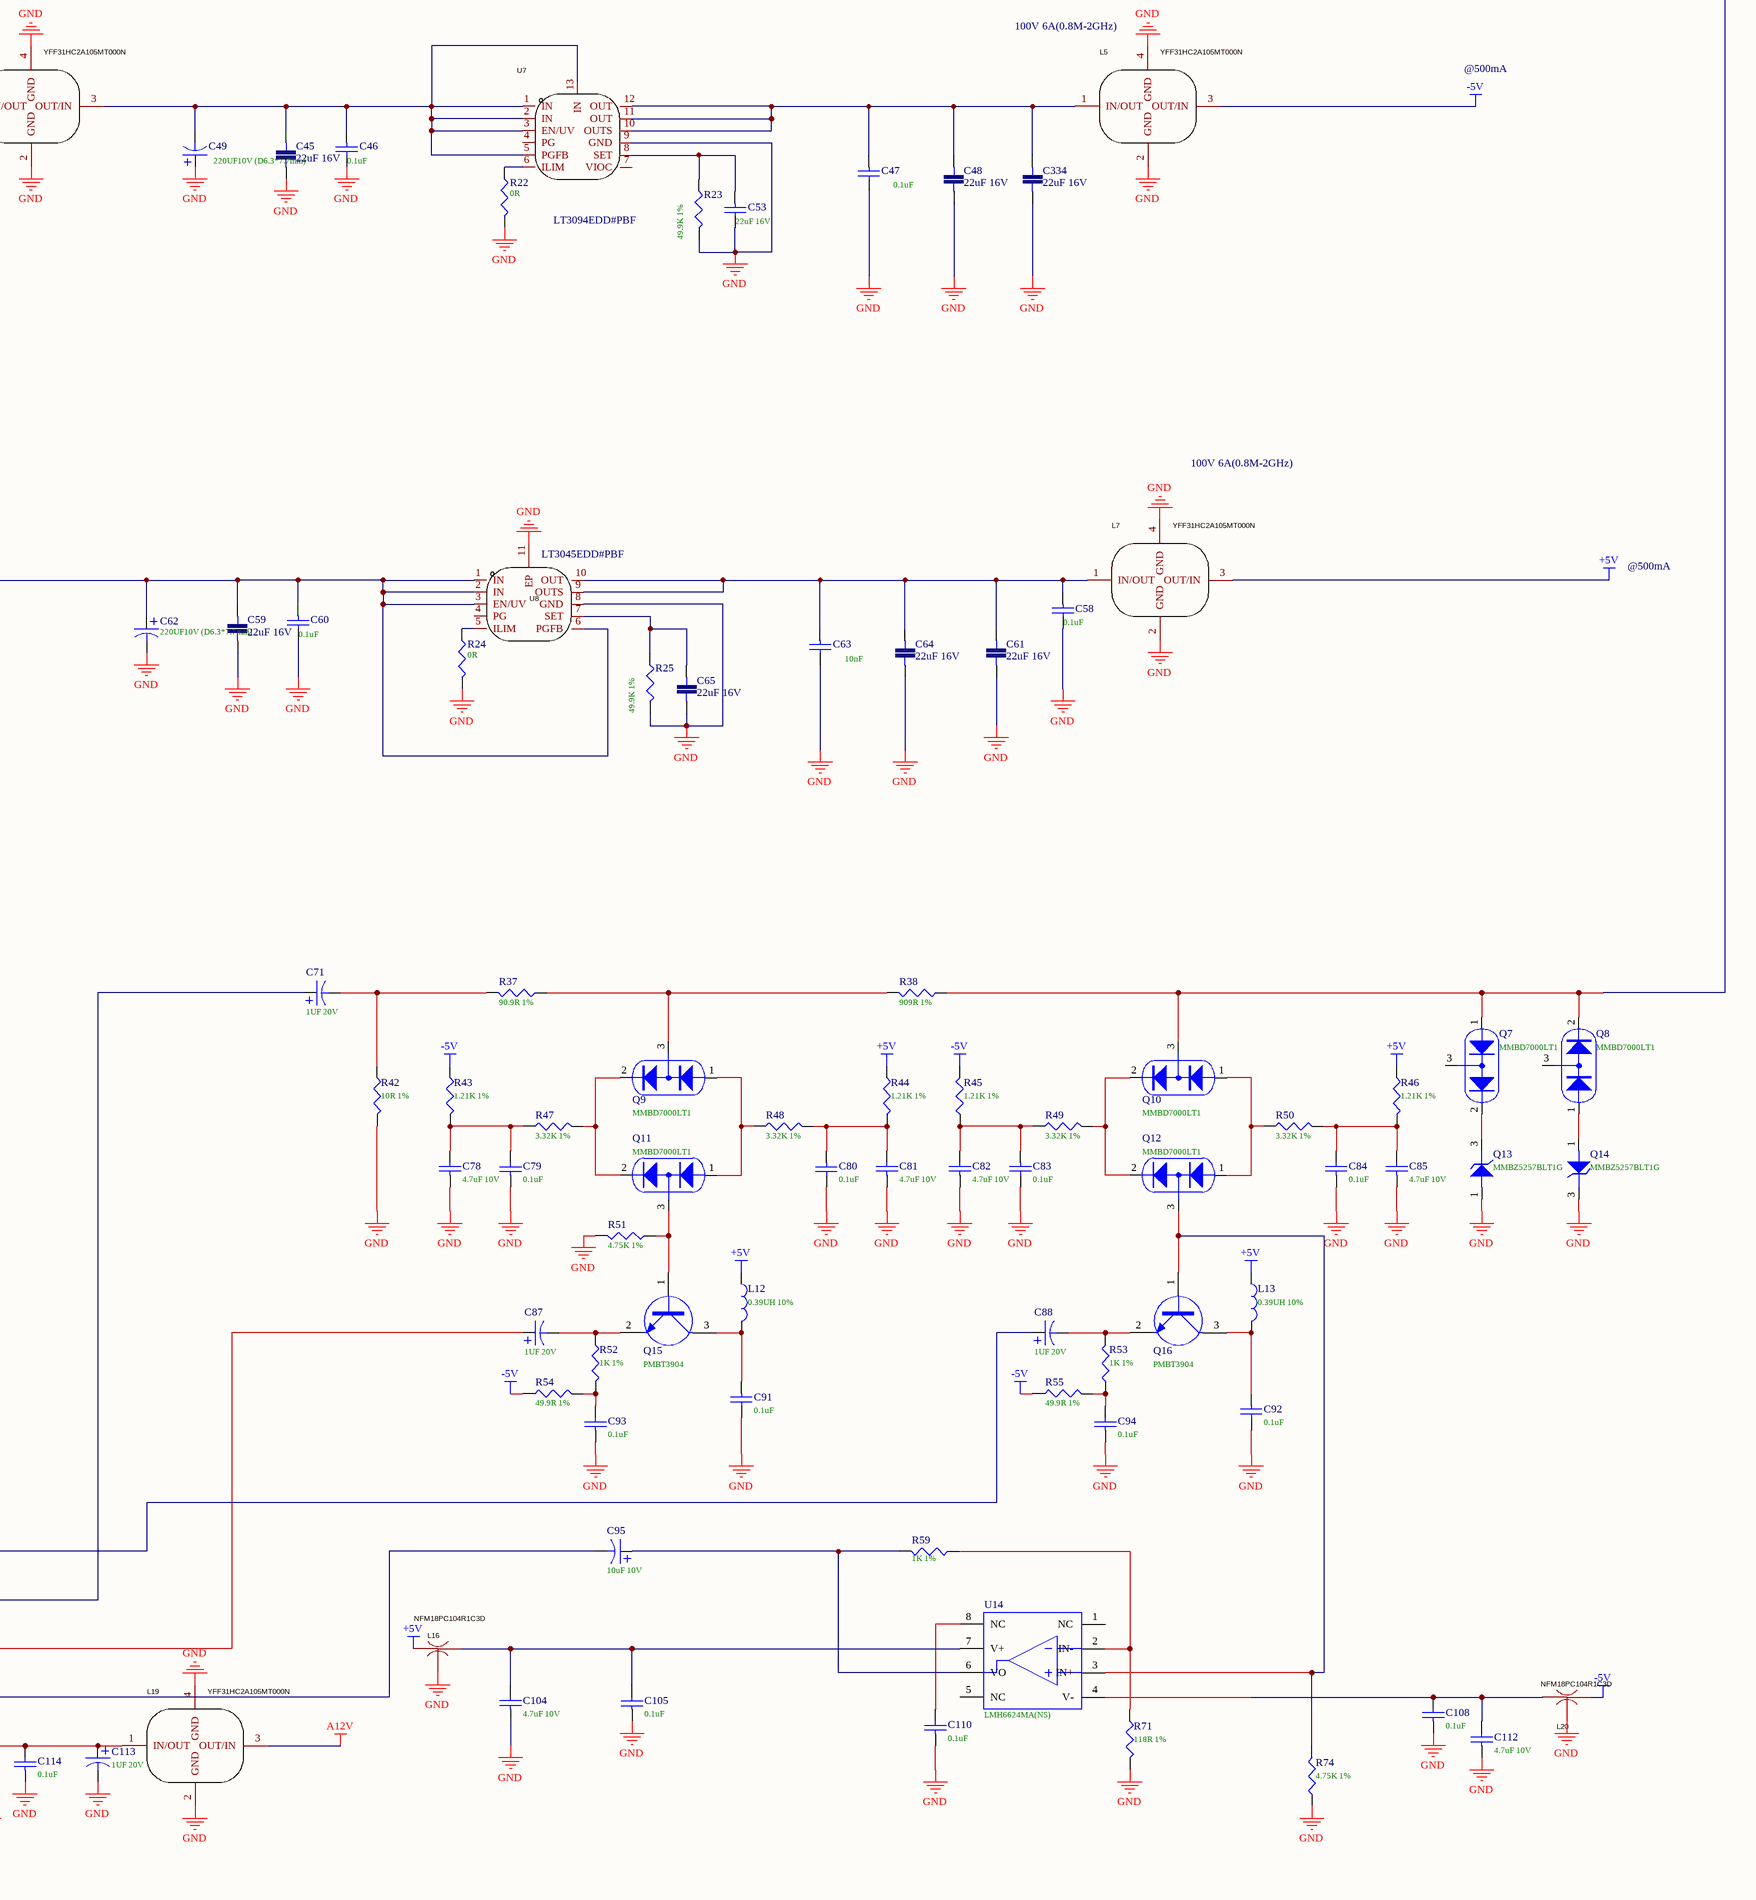
[diagram p0: PCBE109358.SchDoc, bottom column 3 of 4]
# Altium project MISC109358-2.PrjPcb (part 2 of 2)

## Sheet PCBE109358.SchDoc
size 1651 x 889 mm; SheetNumber: 0; SheetTotal: 0

### Parts
1  (no value)  [DIP-1]
+1  (no value)  [DIP-1]
+2  (no value)  [DIP-1]
C3  47uF 25V  [1206]
C4  0.1uF  [0402]
C5  1uF 25V  [0402]
C6  1uF 25V  [0402]
C7  47uF 25V  [1206]
C8  0.1uF  [0402]
C9  1uF 25V  [0402]
C14  0.1uF  [0402]
C15  47uF 25V  [1206]
C16  10uF 10V  [0603]
C17  10uF 10V  [0603]
C18  0.1uF 5% 630V  [AXIAL0.59]
C20  10uF 10V  [0603]
C21  10uF 10V  [0603]
C22  10nF  [0603]
C23  22uF 16V  [0603]
C24  0.1uF  [0603]
C25  0.1uF  [0402]
C26  22uF 16V  [0603]
C27  0.1uF  [0603]
C28  0.1uF  [0402]
C29  47uF 25V  [1206]
C30  47uF 25V  [1206]
C31  4.7uF 25V  [0603]
C32  0.1uF  [0402]
C33  47uF 25V  [1206]
C34  0.1uF  [0402]
C35  4.7uF 25V  [0603]
C36  0.1uF  [0402]
C37  0.1uF  [0402]
C38  4.7uF 10V  [0402]
C39  47uF 25V  [1206]
C40  0.1uF  [0402]
C41  0.1uF  [0402]
C42  47uF 25V  [1206]
C43  0.1uF  [0603]
C45  22uF 16V  [0603]
C46  0.1uF  [0402]
C47  0.1uF  [0402]
C48  22uF 16V  [0603]
C49  220UF10V (D6.3*7.7mm)  [CAP-SMD_BD6.3-L6.6-W6.6-FD]
C50  0.1uF  [0603]
C51  47uF 25V  [1206]
C53  22uF 16V  [0603]
C54  0.1uF  [0603]
C55  47uF 25V  [1206]
C56  2.2UF 10V  [0603钽电容]
C57  10pF  [0402]
C58  0.1uF  [0402]
C59  22uF 16V  [0603]
C60  0.1uF  [0402]
C61  22uF 16V  [0603]
C62  220UF10V (D6.3*7.7mm)  [CAP-SMD_BD6.3-L6.6-W6.6-FD]
C63  10nF  [0402]
C64  22uF 16V  [0603]
C65  22uF 16V  [0603]
C66  4.7uF 10V  [0402]
C67  0.1uF  [0402]
C68  4.7uF 10V  [0402]
C69  0.1uF  [0402]
C70  10nF  [0603]
C71  1UF 20V  [0603钽电容]
C72  NC  [0603]
C73  0.1uF  [0402]
C74  0.1uF  [0402]
C75  4.7uF 10V  [0402]
C76  0.1uF  [0402]
C77  4.7uF 10V  [0402]
C78  4.7uF 10V  [0402]
C79  0.1uF  [0402]
C80  0.1uF  [0402]
C81  4.7uF 10V  [0402]
C82  4.7uF 10V  [0402]
C83  0.1uF  [0402]
C84  0.1uF  [0402]
C85  4.7uF 10V  [0402]
C86  10pF  [0402]
C87  1UF 20V  [0603钽电容]
C88  1UF 20V  [0603钽电容]
C89  4.7uF 10V  [0402]
C90  0.1uF  [0402]
C91  0.1uF  [0402]
C92  0.1uF  [0402]
C93  0.1uF  [0402]
C94  0.1uF  [0402]
C95  10uF 10V  [0603钽电容]
C96  NC  [0603]
C97  0.1uF  [0402]
C98  2.2nF 1%  [0402]
C99  0.1uF  [0402]
C100  4.7uF 10V  [0402]
C101  0.1uF  [0402]
C102  4.7uF 10V  [0402]
C103  2.2nF 1%  [0402]
C104  4.7uF 10V  [0402]
C105  0.1uF  [0402]
C106  1.2nF 1%  [0402]
C107  0.1uF  [0402]
C108  0.1uF  [0402]
C109  2.2UF 10V  [0603钽电容]
C110  0.1uF  [0603]
C111  270pF 1%  [0603]
C112  4.7uF 10V  [0402]
C113  1UF 20V  [0603钽电容]
C114  0.1uF  [0402]
C115  0.1uF  [0402]
C116  0.1uF  [0402]
C117  4.7uF 10V  [0402]
C118  0.1uF  [0402]
C119  100pF 1%  [0603]
C120  4.7uF 10V  [0402]
C121  0.1uF  [0402]
C122  4.7uF 10V  [0402]
C123  4.7uF 10V  [0402]
C124  0.1uF  [0402]
C125  56pF 1%  [0603]
C126  0.1uF  [0402]
C127  4.7uF 10V  [0402]
C128  0.1uF  [0402]
C129  4.7uF 10V  [0402]
C301  0.1uF  [0402]
C302  0.1uF  [0402]
C304  0.1uF  [0402]
C305  4.7uF 10V  [0402]
C306  0.1uF  [0402]
C307  4.7uF 10V  [0402]
C334  22uF 16V  [0603]
D1  ES1D SMA  [1606D]
D2  MMBD914LT1G  [SOT23]
D3  MMBD914LT1G  [SOT23]
D4  ES1D SMA  [1606D]
D5  3SMAJ5929B  [1606D]
D6  DFLU1400-7  [1606D]
D7  ES1D SMA  [1606D]
D8  MMBD914LT1G  [SOT23]
D9  MMBD914LT1G  [SOT23]
D10  MMSZ5248B  [1206D]
D11  MMBZ5231B  [SOT23]
J1  RF connector right-angle socket  [DIP-P]
J2  RF connector right-angle socket  [DIP-P]
K1  TQ2SS-5V(ATQ209SS)SMD10  [K]
K2  TQ2SS-5V(ATQ209SS)SMD10  [K]
K3  TQ2SS-5V(ATQ209SS)SMD10  [K]
K4  TQ2SS-5V(ATQ209SS)SMD10  [K]
L1  YFF31HC2A105MT000N  [FILTER-SMD_4P-L3.2-W1.6-L_YFF31HC]
L2  YFF31HC2A105MT000N  [FILTER-SMD_4P-L3.2-W1.6-L_YFF31HC]
L3  YFF31HC2A105MT000N  [FILTER-SMD_4P-L3.2-W1.6-L_YFF31HC]
L4  YFF31HC2A105MT000N  [FILTER-SMD_4P-L3.2-W1.6-L_YFF31HC]
L5  YFF31HC2A105MT000N  [FILTER-SMD_4P-L3.2-W1.6-L_YFF31HC]
L6  YFF31HC2A105MT000N  [FILTER-SMD_4P-L3.2-W1.6-L_YFF31HC]
L7  YFF31HC2A105MT000N  [FILTER-SMD_4P-L3.2-W1.6-L_YFF31HC]
L8  NFM18PC104R1C3D  [FILTER-SMD_3P-L1.6-W0.8-L_NFM18CC223R1C3D]
L9  NFM18PC104R1C3D  [FILTER-SMD_3P-L1.6-W0.8-L_NFM18CC223R1C3D]
L10  NFM18PC104R1C3D  [FILTER-SMD_3P-L1.6-W0.8-L_NFM18CC223R1C3D]
L11  NFM18PC104R1C3D  [FILTER-SMD_3P-L1.6-W0.8-L_NFM18CC223R1C3D]
L12  0.39UH 10%  [0805]
L13  0.39UH 10%  [0805]
L14  NFM18PC104R1C3D  [FILTER-SMD_3P-L1.6-W0.8-L_NFM18CC223R1C3D]
L15  NFM18PC104R1C3D  [FILTER-SMD_3P-L1.6-W0.8-L_NFM18CC223R1C3D]
L16  NFM18PC104R1C3D  [FILTER-SMD_3P-L1.6-W0.8-L_NFM18CC223R1C3D]
L17  NFM18PC104R1C3D  [FILTER-SMD_3P-L1.6-W0.8-L_NFM18CC223R1C3D]
L18  NFM18PC104R1C3D  [FILTER-SMD_3P-L1.6-W0.8-L_NFM18CC223R1C3D]
L19  YFF31HC2A105MT000N  [FILTER-SMD_4P-L3.2-W1.6-L_YFF31HC]
L20  NFM18PC104R1C3D  [FILTER-SMD_3P-L1.6-W0.8-L_NFM18CC223R1C3D]
L21  NFM18PC104R1C3D  [FILTER-SMD_3P-L1.6-W0.8-L_NFM18CC223R1C3D]
L22  18UH 5%  [0805]
L23  NFM18PC104R1C3D  [FILTER-SMD_3P-L1.6-W0.8-L_NFM18CC223R1C3D]
L24  NFM18PC104R1C3D  [FILTER-SMD_3P-L1.6-W0.8-L_NFM18CC223R1C3D]
L25  10UH 5%  [0805]
L26  NFM18PC104R1C3D  [FILTER-SMD_3P-L1.6-W0.8-L_NFM18CC223R1C3D]
L27  3.9UH 5%  [0805]
L60  NFM18PC104R1C3D  [FILTER-SMD_3P-L1.6-W0.8-L_NFM18CC223R1C3D]
L61  NFM18PC104R1C3D  [FILTER-SMD_3P-L1.6-W0.8-L_NFM18CC223R1C3D]
P1  Header 20X2  [N0.8mm/40Pin-Plug]
P2  Header 4X2  [N0.8mm/8Pin-SOCKET]
P4  Header 20X2  [N0.8mm/40Pin-Plug]
P5  Header 20X2  [N0.8mm/40Pin-Plug]
P6  RF connector straight jack  [DIP-P]
P9  RF connector straight jack  [DIP-P]
Q1  PMBT3904  [SOT23]
Q2  STP10NK80Z  [TO220]
Q3  PMBT3904  [SOT23]
Q4  2N7002-7-F  [SOT23]
Q5  MMBD914LT1G  [SOT23]
Q6  MMBD914LT1G  [SOT23]
Q7  MMBD7000LT1  [SOT23]
Q8  MMBD7000LT1  [SOT23]
Q9  MMBD7000LT1  [SOT23]
Q10  MMBD7000LT1  [SOT23]
Q11  MMBD7000LT1  [SOT23]
Q12  MMBD7000LT1  [SOT23]
Q13  MMBZ5257BLT1G  [SOT23]
Q14  MMBZ5257BLT1G  [SOT23]
Q15  PMBT3904  [SOT23]
Q16  PMBT3904  [SOT23]
Q17  BFT92  [SOT23]
R1  0R  [0402]
R2  470R 5% 1W  [2512]
R3  1K 1W  [2512]
R4  1K 1W  [2512]
R5  2.21K 1%  [0603]
R6  220R 5% 1W  [2512]
R7  10K 1%  [0603]
R8  1.5R  [0603]
R9  1.15K 1%  [1206]
R10  0.5R 1%  [0805]
R11  52.5K 1%  [0603]
R12  1.5R  [0603]
R13  2.21K 1%  [0603]
R14  82R 5% 3W  [2512]
R15  10K 1%  [0603]
R16  10K 1%  [0603]
R17  10K 1%  [0603]
R18  51R 5W  [5W]
R19  13.3K  1%  [0402]
R20  121K  [0603]
R21  0R  [0402]
R22  0R  [0402]
R23  49.9K 1%  [0402]
R24  0R  [0402]
R25  49.9K 1%  [0402]
R26  47R 1%  [0603]
R27  681R 1%  [0603]
R28  22.1K 1%  [0603]
R29  10R 1%  [0603]
R30  100R 1%  [0603]
R31  100R 1%  [0603]
R32  681R 1%  [0603]
R33  0R  [0402]
R34  1K 1%  [0603]
R35  681R 1%  [0603]
R36  100R 1%  [0603]
R37  90.9R 1%  [1206]
R38  909R 1%  [1206]
R39  1.21K 1%  [0603]
R40  5.62K 1%  [0603]
R41  10K 1%  [0603]
R42  10R 1%  [0603]
R43  1.21K 1%  [0603]
R44  1.21K 1%  [0603]
R45  1.21K 1%  [0603]
R46  1.21K 1%  [0603]
R47  3.32K 1%  [0603]
R48  3.32K 1%  [0603]
R49  3.32K 1%  [0603]
R50  3.32K 1%  [0603]
R51  4.75K 1%  [0603]
R52  1K 1%  [0603]
R53  1K 1%  [0603]
R54  49.9R 1%  [0603]
R55  49.9R 1%  [0603]
R56  100R 1%  [0603]
R57  301R 1%  [0603]
R58  20R 1%  [0603]
R59  1K 1%  [0603]
R60  20K 1%  [0603]
R61  20K 1%  [0603]
R62  1K 1%  [0603]
R63  1.21K 1%  [0603]
R64  100R 1%  [0603]
R65  20K 1%  [0603]
R66  1K 1%  [0603]
R67  22.1K 1%  [0603]
R68  0R  [0402]
R69  20K 1%  [0603]
R70  10R 1%  [0603]
R71  118R 1%  [0603]
R72  0R  [0603]
R73  20R 1%  [0603]
R74  4.75K 1%  [0603]
R75  5.62K 1%  [0603]
R76  1K 1%  [0603]
R77  49.9R 1%  [0603]
R78  1.21K 1%  [0603]
R79  10R 1%  [0603]
R800  523K 1%  [0402]
R801  4.7K 1%  [0402]
TP1  (no value)  [TP1]
U1  TPS7A4701RGWR  [QFN-20]
U2  TC4426COA(microchip)  [SO8]
U3  TPL910A  [DFN-8_L3.0-W3.0-P0.65-BL-EP2.3]
U4  TC4426COA(microchip)  [SO8]
U5  GM12051ACPZ-R7  [TDFN-10_L3.0-W3.0-P0.50-BL-EP]
U6  ADR391AUJZ-REEL7  [TSOT-23-5_L2.9-W1.6-P0.95-LS2.8-BR]
U7  LT3094EDD#PBF  [WDFN-12_L3.0-W3.0-P0.45-BL-EP]
U8  LT3045EDD#PBF  [DFN-10_L3.0-W3.0-P0.50-BL-EP]
U9  MASWSS0157TR  [SO8]
U10  AD603AR  [SO8]
U11  AD8002ARZ  [SOP8]
U12  SN74AHC1G04DBVR  [SOT25]
U13  DG540DN PLCC20  [QUAD20]
U14  LMH6624MA(NS)  [SO8]
U15  ADG658YRQZ  [TSSOP-16_L5.0-W4.4-P0.65-LS6.4-TL]
U16  ADG658YRQZ  [TSSOP-16_L5.0-W4.4-P0.65-LS6.4-TL]
U17  AD603AR  [SO8]
U60  AD8002ARZ  [SOP8]

### Nets
12.4V: +2.1 C3.1 C4.1 C5.1 C34.1 C35.1 C54.1 C55.1 L2.3(OUT/IN) P5.31 P5.32 P5.33 P5.34 P5.35 P5.36 P5.37 P5.38 P5.39 P5.40 U1.13(EN) U1.15(IN) U1.16(IN)
+5V: L3.1(IN/OUT) L7.3(OUT/IN) L8.3(OUTPUT) L9.1(INPUT) L12.1 L13.1 L15.1(INPUT) L16.1(INPUT) L17.1(INPUT) L24.3(OUTPUT) L60.3(OUTPUT) R44.1 R46.1 R58.1
-5.4V: +1.1 C42.1 C43.1 L4.1(IN/OUT) P5.1 P5.2 P5.3 P5.4 P5.5 P5.6 P5.7 P5.8 P5.9 P5.10
-5V: L5.3(OUT/IN) L10.1(INPUT) L11.3(OUTPUT) L14.1(INPUT) L18.3(OUTPUT) L20.3(OUTPUT) L21.1(INPUT) L23.1(INPUT) L26.1(INPUT) L61.3(OUTPUT) R43.2 R45.1 R54.2 R55.1 R73.2
A6V: 1.1 C23.2 C24.1 C50.2 C51.1 L6.1(IN/OUT) P5.17 P5.18 P5.19 P5.20 P5.21 P5.22 P5.23 P5.24 U3.5(EN) U3.7(IN) U3.8(IN)
A12V: C30.1 C36.1 C37.1 L19.3(OUT/IN) R801.1 U5.9(OUTS) U5.10(OUT)
GND: C3.2 C4.2 C5.2 C6.2 C7.2 C8.2 C9.2 C14.2 C15.2 C16.1 C17.1 C20.1 C21.1 C23.1 C24.2 C25.2 C26.2 C27.2 C28.2 C29.2 C30.2 C31.2 C32.2 C33.2 C34.2 C35.2 C36.2 C37.2 C38.1 C39.2 C40.1 C41.1 C42.2 C43.2 C45.1 C46.2 C47.2 C48.1 C49.1 C50.1 C51.2 C53.2 C54.2 C55.2 C57.1 C58.2 C59.1 C60.2 C61.1 C62.2 C63.2 C64.1 C65.1 C66.1 C67.2 C68.1 C69.2 C72.2 C73.2 C74.2 C75.1 C76.2 C77.1 C78.1 C79.1 C80.2 C81.1 C82.1 C83.2 C84.1 C85.1 C86.2 C89.1 C90.2 C91.2 C92.2 C93.1 C94.1 C96.2 C97.1 C99.1 C100.1 C101.2 C102.1 C103.1 C104.1 C105.1 C108.1 C110.1 C112.1 C113.2 C114.1 C115.2 C116.1 C117.1 C118.1 C120.1 C121.1 C122.1 C123.1 C124.2 C126.1 C127.1 C128.1 C129.1 C301.2 C302.1 C304.2 C305.1 C306.2 C307.1 C334.1 D10.1(A) J1.1 J1.2 J1.3 J1.4 J2.1 J2.2 J2.3 J2.4 K1.3 K1.8 K2.4 K2.7 K3.3 K3.8 K4.4 K4.7 L1.2(GND) L1.4(GND) L2.2(GND) L2.4(GND) L3.2(GND) L3.4(GND) L4.2(GND) L4.4(GND) L5.2(GND) L5.4(GND) L6.2(GND) L6.4(GND) L7.2(GND) L7.4(GND) L8.2(GND) L9.2(GND) L10.2(GND) L11.2(GND) L14.2(GND) L15.2(GND) L16.2(GND) L17.2(GND) L18.2(GND) L19.2(GND) L19.4(GND) L20.2(GND) L21.2(GND) L23.2(GND) L24.2(GND) L26.2(GND) L60.2(GND) L61.2(GND) P1.5 P1.6 P1.11 P1.12 P1.17 P1.18 P1.20 P1.23 P1.24 P1.29 P1.30 P1.35 P1.36 P2.1 P2.3 P2.5 P2.7 P4.5 P4.6 P4.11 P4.12 P4.17 P4.18 P4.23 P4.24 P4.29 P4.30 P4.35 P4.36 P5.11 P5.12 P5.13 P5.14 P5.15 P5.16 P5.25 P5.26 P5.27 P5.28 P5.29 P5.30 P6.1 P6.2 P6.3 P6.4 P9.1 P9.2 P9.3 P9.4 Q1.2(E) Q3.2(E) Q4.2(S) Q5.3(K) Q6.1(A) Q13.1(A) Q14.3(K) R2.2 R7.2 R9.2 R10.1 R15.2 R16.2 R17.1 R19.2 R20.2 R21.2 R22.2 R23.2 R24.2 R25.2 R34.2 R35.2 R36.2 R39.2 R40.1 R41.1 R42.1 R51.2 R60.1 R61.2 R63.1 R65.2 R66.1 R69.1 R71.1 R74.1 R75.1 R78.2 U1.5(6P4V1) U1.6(3P2V) U1.7(GND) U1.9(0P8V) U1.11(0P2V) U1.21(EPAD) U2.3(GND) U3.4(GND) U3.9(pad) U4.3(GND) U5.8(GND) U5.11(EP) U6.5(GND) U7.9(GND) U8.8(GND) U8.11(EP) U9.2(GND) U9.7(GND) U9.8(GND) U10.4(COMM) U12.5(VCC) U13.3(GND) U13.6(GND) U13.8(GND) U13.13(GND) U13.15(GND) U13.18(GND) U15.6(EN#) U15.8(GND) U16.6(EN#) U16.8(GND) U17.4(COMM)
H5V: C16.2 C17.2 C20.2 C21.2 C22.2 C25.1 C26.1 D2.3(K) D3.3(K) D8.3(K) D9.3(K) K1.1 K2.1 K3.1 K4.1 R11.2 TP1.1 U3.1(OUT) U3.2(OUT)
H12V: C7.1 C8.1 C9.1 D1.2(K) L1.1(IN/OUT) R1.1 U1.1(OUT) U1.20(OUT)
VREF: C38.2 C41.2 R28.1 R67.2 U6.3(VOUT/SENSE) U6.4(VOUT/FORCE)
AK1: P1.27 Q4.1(G) R17.2
AK10: P1.19 R13.2
AK13: P1.21 R5.2
AS27: P4.38
AS28: P4.40
Attn1: P4.34
Attn2: P4.32
Attn4: P4.28
Attn8: P4.26
Attn16: P4.22
DAC Clk: P4.14
DAC Data: P4.16
DAC Strobe: P4.10
GPOS1: C72.1 C96.1 R56.1 U10.1(GPOS) U17.1(GPOS)
HP Filt En: P4.4
HT: P2.2 P2.4 P2.6 P2.8 R3.2
IN1: P4.20
IN2: P4.8
K0: D11.3(K) P4.9
LB_A0: P4.27 U15.9(A2)
LB_A1: P4.25 U15.10(A1)
LB_A2: P4.21 U15.11(A0)
LB_A4: P4.19 U16.9(A2)
LB_A5: P4.15 U16.10(A1)
LB_A6: P4.13 U16.11(A0)
LB_IN1: R72.1 U15.13(S1)
LB_IN2: R77.2 U15.14(S2)
LB_IN3: R79.2 U15.15(S3)
LB_IN4: R68.1 U15.12(S4)
LB_OUT: R33.1 R41.2 U16.3(D)
LP Filt En: P4.2
TT: P1.22 R9.1 U2.2(IN_A) U2.4(IN_B) U4.2(IN_A) U4.4(IN_B)
U15_IN1: P4.39 R61.1 U13.20(IN2)
U15_IN2: P4.37 R60.2 U13.1(IN1)
U15_IN3: P4.33 R65.1 U13.11(IN3)
U15_IN4: P4.31 R69.2 U13.10(IN4)
NetC6_1: C6.1 U1.14(NR)
NetC14_1: C14.1 C15.1 C28.1 C29.1 L1.3(OUT/IN) U2.6(VDD) U4.6(VDD)
NetC18_1: C18.1 Q2.2(D) R4.2
NetC18_2: C18.2 D5.2(K) D6.2(K)
NetC22_1: C22.1 R11.1 R15.1 U3.3(FB)
NetC27_1: C27.1 U3.6(RN)
NetC31_1: C31.1 R20.1 U5.7(SET)
NetC32_1: C32.1 C33.1 L2.1(IN/OUT) U5.1(IN) U5.2(IN) U5.3(EN/UV)
NetC39_1: C39.1 C40.2 L3.3(OUT/IN) U6.1(SHDN#) U6.2(VIN)
NetC45_2: C45.2 C46.1 C49.2 L4.3(OUT/IN) U7.1(IN) U7.2(IN) U7.3(EN/UV) U7.5(PGFB) U7.13(IN)
NetC47_1: C47.1 C48.2 C334.2 L5.1(IN/OUT) U7.10(OUTS) U7.11(OUT) U7.12(OUT)
NetC53_1: C53.1 R23.1 U7.8(SET)
NetC56_1: C56.1 C57.2 P6.5
NetC56_2: C56.2 Q5.1(A) Q6.3(K) R26.2
NetC58_1: C58.1 C61.2 C63.1 C64.2 L7.1(IN/OUT) U8.9(OUTS) U8.10(OUT)
NetC59_2: C59.2 C60.1 C62.1 L6.3(OUT/IN) U8.1(IN) U8.2(IN) U8.3(EN/UV) U8.6(PGFB)
NetC65_2: C65.2 R25.1 U8.7(SET)
NetC66_2: C66.2 C67.1 L8.1(INPUT) U11.8(V+)
NetC68_2: C68.2 C69.1 L9.3(OUTPUT) U10.8(VPOS)
NetC70_1: C70.1 R39.1 U9.3(RF1)
NetC70_2: C70.2 R29.1
NetC71_1: C71.1 U13.17(S2)
NetC71_2: C71.2 R37.1 R42.2
NetC73_1: C73.1 R28.2 R40.2 U10.2(GNEG)
NetC74_1: C74.1 C75.2 L10.3(OUTPUT) U10.6(VNEG)
NetC76_1: C76.1 C77.2 L11.1(INPUT) U11.4(V-)
NetC78_2: C78.2 C79.2 R43.1 R47.2
NetC80_1: C80.1 C81.2 R44.2 R48.1
NetC82_2: C82.2 C83.1 R45.2 R49.1
NetC84_2: C84.2 C85.2 R46.2 R50.2
NetC86_1: C86.1 U9.4(A) U12.4(Y)
NetC87_1: C87.1 U13.14(S3)
NetC87_2: C87.2 Q15.2(E) R52.1
NetC88_1: C88.1 U13.4(S1)
NetC88_2: C88.2 Q16.2(E) R53.2
NetC89_2: C89.2 C90.1 L14.3(OUTPUT) U12.3(GND)
NetC91_1: C91.1 L12.2 Q15.3(C)
NetC92_1: C92.1 L13.2 Q16.3(C)
NetC93_2: C93.2 R52.2 R54.1
NetC94_2: C94.2 R53.1 R55.2
NetC95_1: C95.1 R59.2 U14.6(VO)
NetC95_2: C95.2 U13.7(S4)
NetC97_2: C97.2 R57.2 R58.2
NetC98_1: C98.1 C106.1 U16.15(S3)
NetC98_2: C98.2 C103.2 C106.2 R68.2
NetC99_2: C99.2 C102.2 L17.3(OUTPUT) U17.8(VPOS)
NetC100_2: C100.2 C101.1 L15.3(OUTPUT) R62.2
NetC104_2: C104.2 C105.2 L16.3(OUTPUT) U14.7(V+)
NetC107_1: C107.1 U15.3(D)
NetC107_2: C107.2 R70.2
NetC108_2: C108.2 C112.2 L20.1(INPUT) U14.4(V-)
NetC109_1: C109.1 Q17.2(E) R57.1
NetC109_2: C109.2 U17.3(VINP)
NetC110_2: C110.2 U14.8(NC)
NetC111_1: C111.1 L22.1
NetC111_2: C111.2 R72.2
NetC113_1: C113.1 C114.2 L19.1(IN/OUT) U13.16(V+)
NetC115_1: C115.1 R67.1 R75.2 U17.2(GNEG)
NetC116_2: C116.2 C117.2 Q17.3(C) R73.1
NetC118_2: C118.2 C120.2 L21.3(OUTPUT) U13.5(V-)
NetC119_1: C119.1 L25.1
NetC119_2: C119.2 R77.1
NetC121_2: C121.2 C122.2 L26.3(OUTPUT) U17.6(VNEG)
NetC123_2: C123.2 C124.1 L23.3(OUTPUT) U16.7(VSS)
NetC125_1: C125.1 L27.1
NetC125_2: C125.2 R79.1
NetC126_2: C126.2 C129.2 L24.1(INPUT) R76.2
NetC127_2: C127.2 C128.2 L18.1(INPUT) U15.7(VSS)
NetC301_1: C301.1 R62.1 R63.2 U16.16(VDD)
NetC302_2: C302.2 R76.1 R78.1 U15.16(VDD)
NetC304_1: C304.1 C305.2 L61.1(INPUT) U60.4(V-)
NetC306_1: C306.1 C307.2 L60.1(INPUT) U60.8(V+)
NetD1_1: D1.1(A) D4.2(K)
NetD2_1: D2.1(A) K1.10 Q1.3(C)
NetD3_1: D3.1(A) D9.1(A) K2.10 K4.10 Q4.3(D)
NetD4_1: D4.1(A) D5.1(A)
NetD6_1: D6.1(A) D7.2(K)
NetD7_1: D7.1(A) J1.5 K2.2 K2.9 R2.1 R6.2 R14.2
NetD8_1: D8.1(A) K3.10 Q3.3(C)
NetD10_2: D10.2(K) Q2.1(G) R8.1 R12.1
NetD11_1: D11.1(A) U12.2(A)
NetJ2_5: J2.5 K4.2 K4.9 R18.1
NetK1_4: K1.4 K1.7 R6.1
NetK2_3: K2.3 K2.8 K4.3 K4.8
NetK3_4: K3.4 K3.7 R14.1
NetL22_2: L22.2 U16.14(S2)
NetL25_2: L25.2 U16.13(S1)
NetL27_2: L27.2 U16.12(S4)
NetP9_5: P9.5 R56.2
NetQ1_1: Q1.1(B) R5.1 R7.1
NetQ2_3: Q2.3(S) R10.2
NetQ3_1: Q3.1(B) R13.1 R16.1
NetQ7_1: Q7.1 Q8.2 Q10.3 R18.2 R38.2
NetQ7_2: Q7.2 Q13.3(K)
NetQ8_1: Q8.1 Q14.1(A)
NetQ9_1: Q9.1 Q11.1 R48.2
NetQ9_2: Q9.2 Q11.2 R47.1
NetQ9_3: Q9.3 R37.2 R38.1
NetQ10_1: Q10.1 Q12.1 R50.1
NetQ10_2: Q10.2 Q12.2 R49.2
NetQ11_3: Q11.3 Q15.1(B) R51.1
NetQ12_3: Q12.3 Q16.1(B) R74.2 U14.3(IN+)
NetQ17_1: Q17.1(B) R64.1
NetR1_2: R1.2 U1.3(SENSE/FB)
NetR3_1: R3.1 R4.1
NetR8_2: R8.2 U2.7(~{OUTA}) U4.7(~{OUTA})
NetR12_2: R12.2 U2.5(~{OUTB}) U4.5(~{OUTB})
NetR19_1: R19.1 R800.2 U5.6(PGFB)
NetR21_1: R21.1 U5.5(ILIM)
NetR22_1: R22.1 U7.6(ILIM)
NetR24_1: R24.1 U8.5(ILIM)
NetR26_1: R26.1 R27.1 U60.1(OUT1)
NetR27_2: R27.2 R35.1 U60.2(-IN1)
NetR29_2: R29.2 R32.1 U11.7(OUT2)
NetR30_1: R30.1 U60.3(+IN1)
NetR30_2: R30.2 R34.1 U9.1(RFC)
NetR31_1: R31.1 U11.5(+IN2)
NetR31_2: R31.2 U10.5(FDBK) U10.7(VOUT)
NetR32_2: R32.2 R36.1 U11.6(-IN2)
NetR33_2: R33.2 U10.3(VINP)
NetR59_1: R59.1 R71.2 U14.2(IN-)
NetR64_2: R64.2 R66.2 U13.2(D1) U13.9(D4) U13.12(D3) U13.19(D2)
NetR70_1: R70.1 U17.5(FDBK) U17.7(VOUT)
NetR800_1: R800.1 R801.2

Not connected (* = marked no-connect by the designer): K1 2 5 6 9; K2 5 6; K3 2 5 6 9; K4 5 6; P1 1 2 3 4 7 8 9 10 13 14 15 16 25 26 28 31 32 33 34 37 38 39 40; P4 1 3 7; Q7 3; Q8 3; U1 2(NC) 4(6P4V2) 8(1P6V) 10(0P4V) 12(0P1V) 17(NC) 18(NC) 19(NC); U2 1(NC) 8(NC); U4 1(NC) 8(NC); U5 4(PG); U7 4(PG) 7(VIOC); U8 4(PG); U9 5(B) 6(RF2); U11 1(OUT1) 2(-IN1) 3(+IN1); U14 1(NC) 5(NC); U15 1(S5) 2(S7) 4(S8) 5(S6); U16 1(S5) 2(S7) 4(S8) 5(S6); U60 5(+IN2) 6(-IN2) 7(OUT2)

### Notes on the sheet
- @1A
- (near P2) 500V high-voltage interface
- transmit interface
- (near U2) negative pulse
- (near R7) separate shield ring
- receive interface
- Couts connected to output capacitor and load
- (near L5) 100V 6A(0.8M-2GHz)
- @500mA
- 100V 6A(0.8M-2GHz)
- (near R68) 0.25MHz--2.25MHz
- tentative 2-10MHZ
- 2.25MHz
- (near R77) tentative 10-30MHZ
- (near R77) 5MHz
- (near R79) 10MHz(7.5--14.5MHz)
- Title
- Size:
- Date:
- File:
- A0
- Number:
- Time:
- Revision:
- Sheet
- of

### Library data of the parts
1 +1 +2 = TP
C3-C9 C14-C18 C20 C21 C28-C43 C46 C47 C50 C51 C53-C55 C57 C58 C60 C63 C66-C70 C72-C86 C89-C94 C96-C108 C110-C112 C114-C129 C301 C302 C304-C307 = CAP: Capacitor
C22 C23 C25 C26 C45 C48 C59 C61 C64 C65 C334 = C1206
C24 C27 = C0402
C49 C62 = CAPACITOR_1: Capacitor
C56 C71 C87 C88 C95 C109 C113 = CAPACITOR
D1 D4 D6 D7 = DIODE
D5 D10 = ZENER3: Zener Diode
D11 = MMBZ5257BLT1G
J1 J2 P6 P9 = JA1
K1-K4 = TQ2SS-5V
L1-L7 L19 = YFF31HC2A105MT000N: Manufacturer: TDK; Add into BOM: yes; Nominal Capacitance: 1uF; CapacitanceTolerance: ±20%; DC Rated Voltage: 100V; Rated Current: 6A; DC Resistance: 5mΩ; Name: YFF31HC2A105MT000N; Symbol: YFF31HC2A105MT000N; Device: YFF31HC2A105MT000N; LCSC Part Name: 1uF(105) ±20% 100V; Supplier Part: C113216; Manufacturer Part: YFF31HC2A105MT000N; Supplier Footprint: SMD-4P,1.6x3.2mm; JLCPCB Part Class: Extended Part; Datasheet: https://example.com/upload/public/pdf/source/20180326/C113216_F6F81E50B9805DA3D7C436129903DEBD.pdf; Supplier: LCSC; Convert to PCB: yes; Operating Temperature: -55℃~+125℃
L8-L11 L14-L18 L20 L21 L23 L24 L26 L60 L61 = NFM15PC104R1A3D: Manufacturer: muRata(村田); Add into BOM: yes; Nominal Capacitance: 100nF; CapacitanceTolerance: ±20%; DC Rated Voltage: 10V; Rated Current: 2A; DC Resistance: 30mΩ; Symbol: NFM15PC104R1A3D; Device: NFM15PC104R1A3D; LCSC Part Name: 0.1uF ±20% 10V; Supplier Part: C2650905; Manufacturer Part: NFM15PC104R1A3D; Supplier Footprint: 0402; JLCPCB Part Class: Extended Part; Datasheet: https://example.com/upload/public/pdf/source/20210611/05FD8D968916F804F398094FB2B4AAFE.pdf; Supplier: LCSC; Convert to PCB: yes; Operating Temperature: -55℃~+105℃; Comment_1: NFM15PC104R1A3D
L12 L13 L22 L25 L27 = INDUCTOR
P1 P4 P5 = Header 20X2: Header, 20-Pin, Dual row; LatestRevisionDate: 17-Jul-2002; LatestRevisionNote: Re-released for DXP Platform.; Publisher: Altium Limited
P2 = Header 4X2: Header, 4-Pin, Dual row; LatestRevisionDate: 17-Jul-2002; LatestRevisionNote: Re-released for DXP Platform.; Publisher: Altium Limited
Q1 Q3 Q15 Q16 = NPN: NPN Transistor
Q7-Q12 = D1: Diode
Q13 Q14 = MMBZ5231B
Q17 = PNP: PNP Transistor
R1 R20 R33 R68 R72 = RES
R2-R10 R12-R14 R16-R19 R21-R32 R34-R67 R69-R71 R73-R79 R800 R801 = RES1
R11 R15 = R0603: Value: NM
TP1 = TEST_2
U1 = TPS7A4701RGWR(QFN20): Name: *; Symbol: *; Device: *; LCSC Part Name: *; Supplier Part: *; Manufacturer: *; Manufacturer Part: *; Supplier Footprint: *; JLCPCB Part Class: *; Datasheet: *; Supplier: *; Add into BOM: *; Convert to PCB: *; Output Type: *; Output Polarity: *; Number of Outputs: *
U2 U4 = TC4426COA
U3 = TPL910A: 3PEAK
U5 = GM12051ACPZ-R7: Manufacturer: GONGMOSEMI(共模半导体); Add into BOM: yes; Output Type: Output Type text   adjustable; Maximum Input Voltage: 20V; Output Voltage: 1V~15V; Output Current: 1A; Power Supply Rejection Ratio (PSRR): 98dB@(10kHz);59dB@(2MHz); Noise: 1.8uVrms; Symbol: GM12051ACPZ-R7; Device: GM12051ACPZ-R7; LCSC Part Name: 输入20V 输出可调 1A; Supplier Part: C7452155; Manufacturer Part: GM12051ACPZ-R7; Supplier Footprint: DFN-10-EP(3x3); JLCPCB Part Class: Extended Part; Datasheet: https://example.com/upload/public/pdf/source/20240521/A461AE2845FB763CD11E4AE852B5A4F1.pdf; Supplier: LCSC; Convert to PCB: yes; Dropout Voltage: -; standby current: -; Feature: -; Operating Temperature: -; Output Polarity: -; Number of Outputs: -; Comment_1: GM12051ACPZ-R7
U6 = ADR391AUJZ-REEL7: Manufacturer: ADI(亚德诺); Add into BOM: yes; Output Type: Output Type text   fixed; Input Voltage: 2.8V~15V; Output Voltage: 2.5V; Output Current: 5mA; Tolerance: ±0.24%; Temperature Coefficient: 25ppm/℃; Reference Type: Reference Type tex series; Supply Current: 140uA; Symbol: ADR391AUJZ-REEL7; Device: ADR391AUJZ-REEL7; LCSC Part Name: ADR391AUJZ-REEL7; Supplier Part: C141376; Manufacturer Part: ADR391AUJZ-REEL7; Supplier Footprint: TSOT-23-5; JLCPCB Part Class: Extended Part; Datasheet: https://example.com/upload/public/pdf/source/20180613/C206648_9731C7AF92F4D28594246B6DF6883AF4.pdf; Supplier: LCSC; Convert to PCB: yes; Operating Temperature: -40℃~+125℃@(TA); Comment_1: ADR391AUJZ-REEL7
U7 = LT3094EDD#PBF: Add into BOM: yes; Symbol: LT3094EDD#PBF; Device: LT3094EDD#PBF; LCSC Part Name: LT3094EDD#PBF; Supplier Part: C670492; Manufacturer Part: LT3094EDD#PBF; Supplier Footprint: WDFN-12-EP(3x3); JLCPCB Part Class: Extended Part; Datasheet: https://example.com/upload/public/pdf/source/20200318/C498217_A5485280C797CF3891C55BEBE66C21D4.pdf; Supplier: LCSC; Convert to PCB: yes; Output Type: -
U8 = LT3045EDD#PBF: Symbol: LT3045EDD#PBF_C666574; Add into BOM: yes; Maximum Input Voltage: 20V; Output Voltage: 0V~15V; MAX Output Current: 500mA; Dropout Voltage: 450mV@(500mA); standby current: 20uA; Number of Outputs: 1; Device: LT3045EDD#PBF; LCSC Part Name: LT3045EDD#PBF; Supplier Part: C666574; Manufacturer Part: LT3045EDD#PBF; Supplier Footprint: DFN-10-EP(3x3); JLCPCB Part Class: Extended Part; Datasheet: https://example.com/upload/public/pdf/source/20200416/C514420_E440C492D6C74EAE6AB301243586F696.pdf; Supplier: LCSC; Convert to PCB: yes
U11 U60 = AD8002ARZ: Manufacturer: ADI(亚德诺); Add into BOM: yes; Number of Circuits: Number of Circuits dual; Current - Input Bias(Ib): 5uA; Slew Rate(SR): 1200V/us; Output Current: 70mA; -3db Bandwidth: 600MHz; Symbol: AD8002ARZ; Device: AD8002ARZ; LCSC Part Name: AD8002ARZ; Supplier Part: C652147; Manufacturer Part: AD8002ARZ; Supplier Footprint: SOIC-8; JLCPCB Part Class: Extended Part; Datasheet: https://example.com/upload/public/pdf/source/20200709/C652144_DEB46A3C7F92B3B6140B45EB30A5CF9A.pdf; Supplier: LCSC; Convert to PCB: yes; Gain Bandwidth Product(GBP): -; Operating Temperature: -40℃~+85℃; Comment_1: AD8002ARZ
U13 = DG540DN
U14 = LMH6624MA